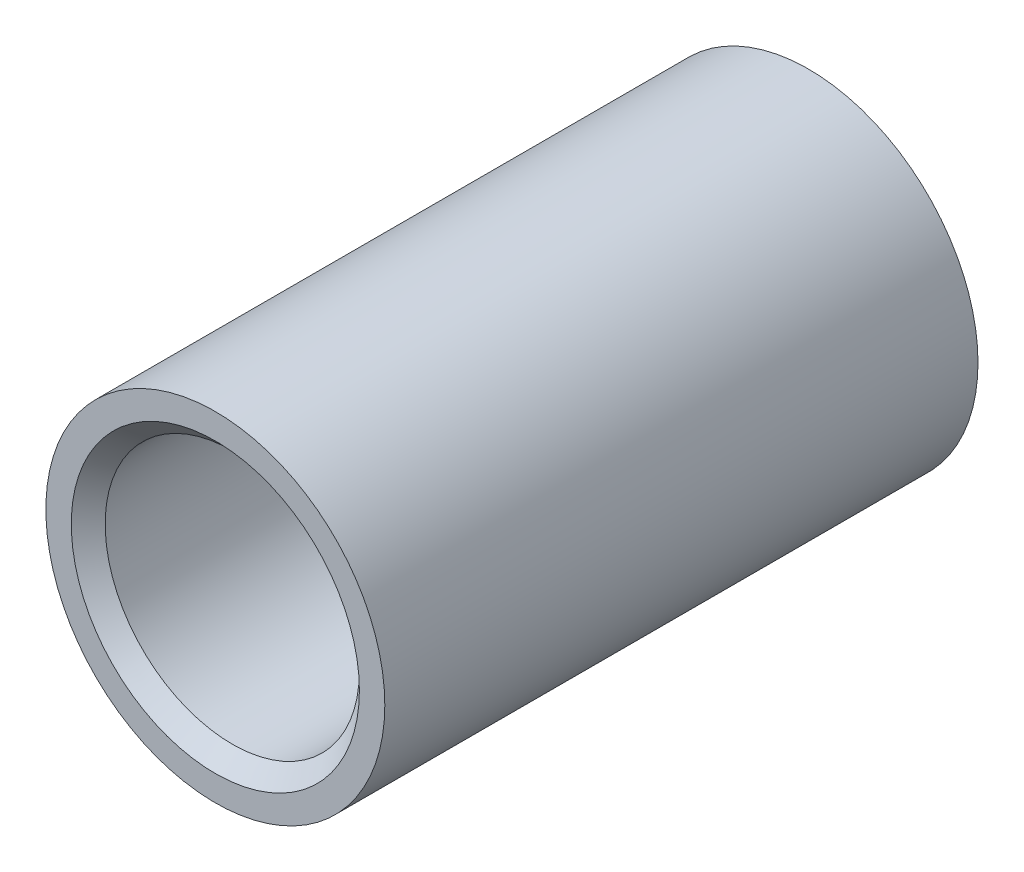
from build123d import *

# Parameters (mm, degrees)
SKETCH1_R           = 10
SKETCH1_R_2         = 7.5
BOSS_EXTRUDE1_DEPTH = 35
CHAMFER1_SIZE       = 1


with BuildPart() as part:
    # Sketch1 → Boss-Extrude1 (new body)
    with BuildSketch(Plane.XY):
        Circle(SKETCH1_R)
        Circle(SKETCH1_R_2, mode=Mode.SUBTRACT)
    extrude(amount=BOSS_EXTRUDE1_DEPTH)

    # Chamfer1
    chamfer1_edges = [part.edges().sort_by_distance(p)[0] for p in [
        (-7.5, 0, 0),
        (-7.5, 0, 35),
    ]]
    chamfer(chamfer1_edges, length=CHAMFER1_SIZE)


solid = part.part
